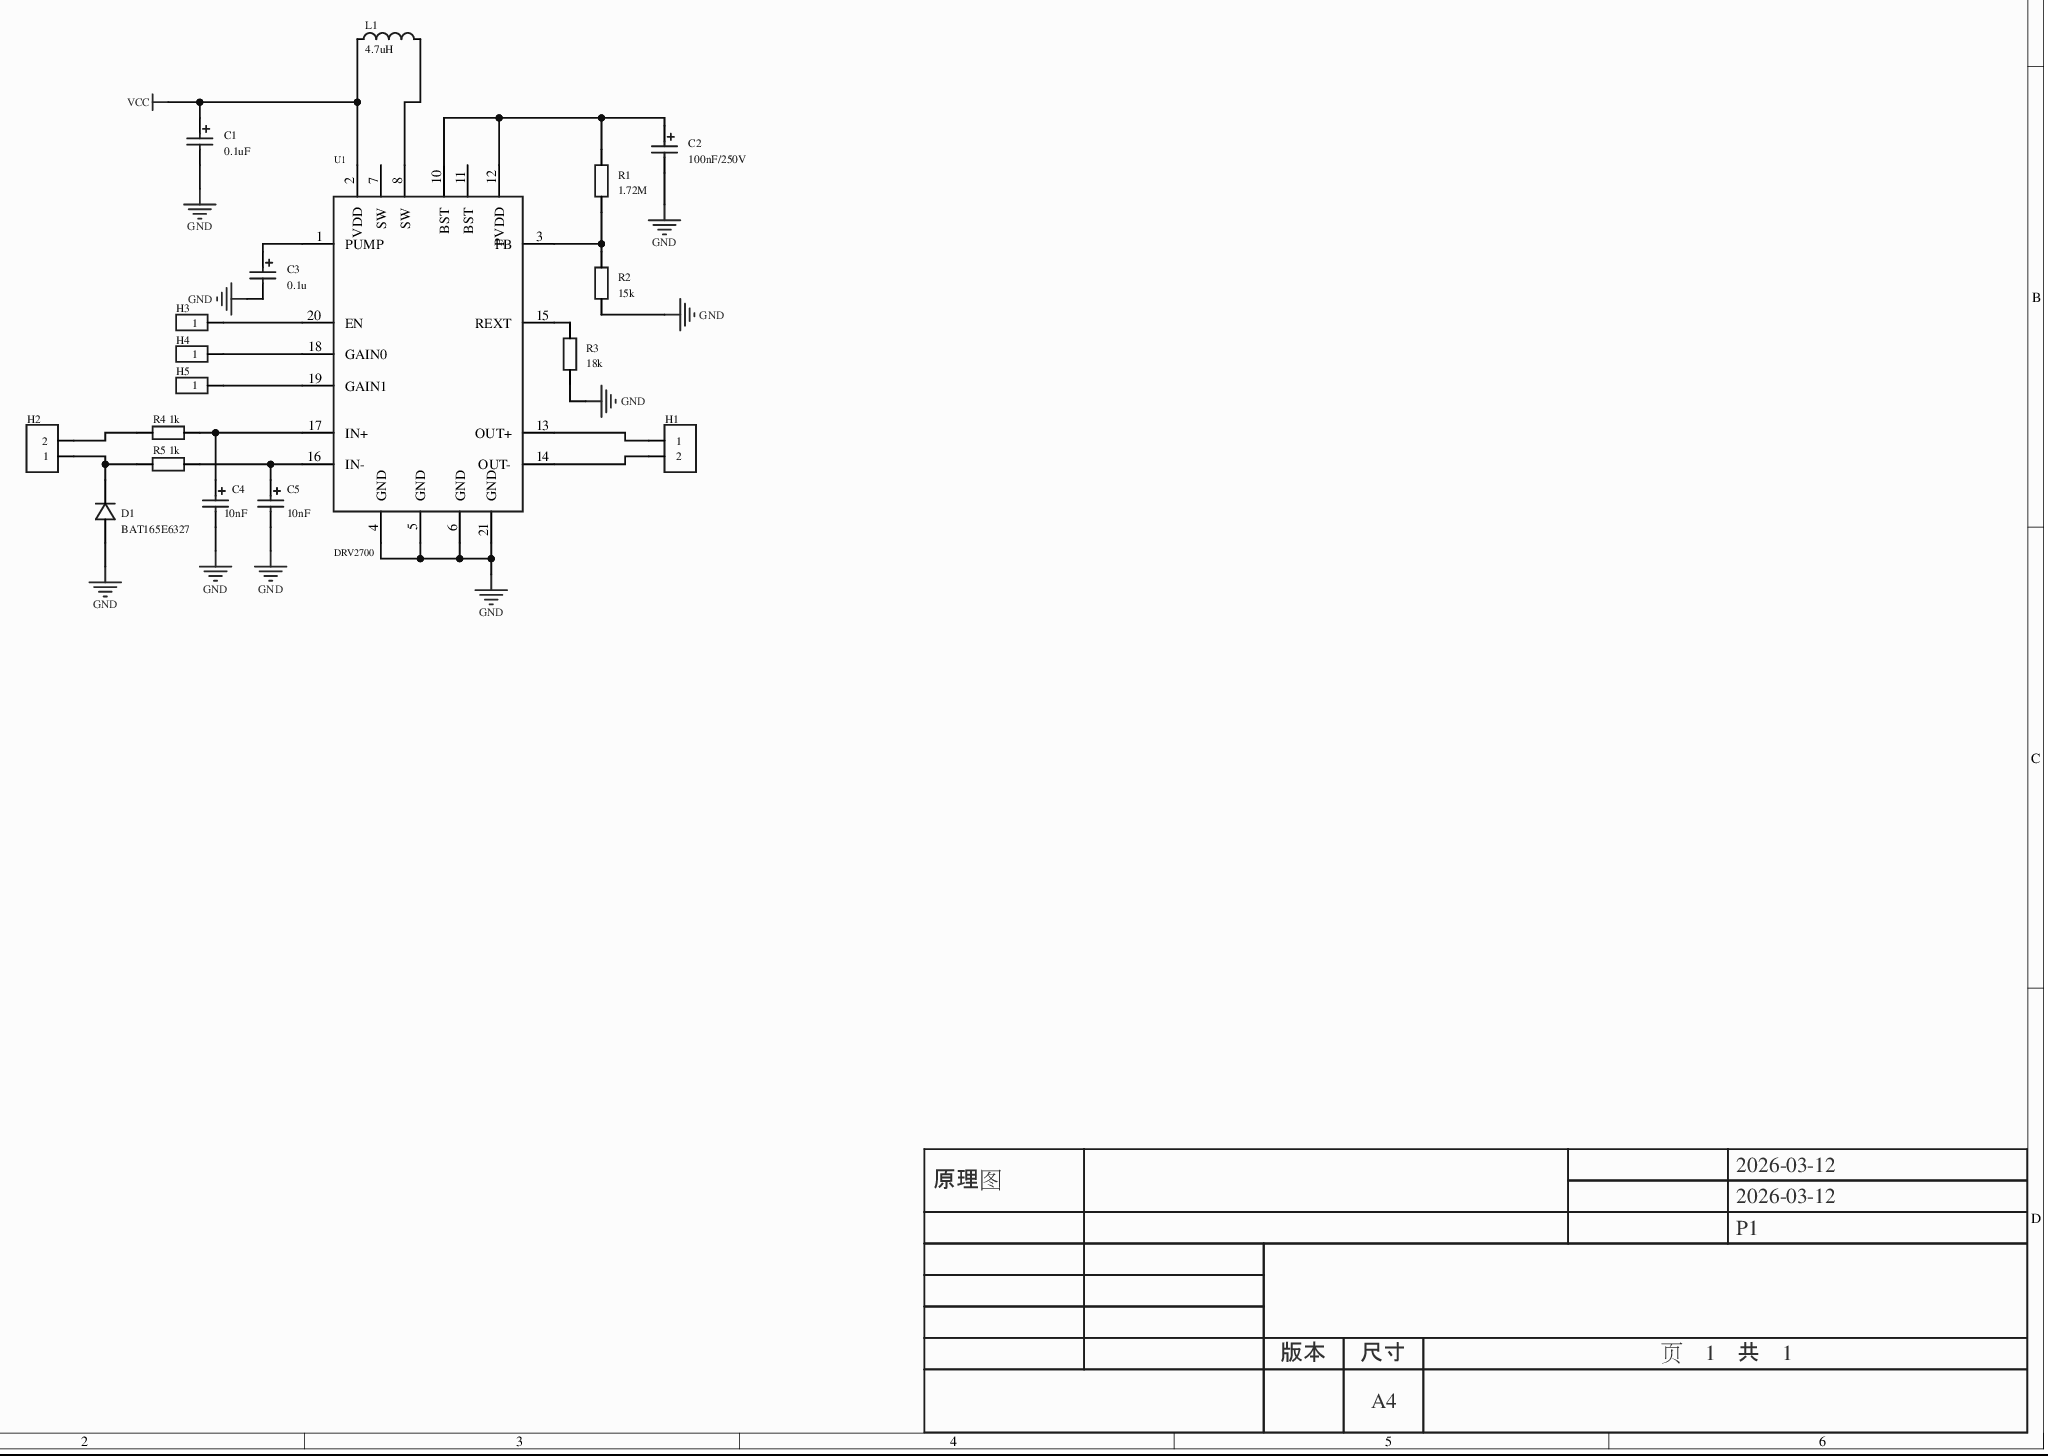
[diagram p0: MISC50934-3.schdoc]
# Altium project MISC50934-2.PrjPcb
1 sheet, 18 parts. Net scope: global (net labels, ports and power ports of the same name join across sheets).
Board file: MISC50934.pcbdoc

## Sheet MISC50934-3.schdoc
size 420 x 297 mm; Version: V1.0; @Project Name: MISC50934; @Update Date: 2026-03-12; @Create Date: 2026-03-12; @Board Name: MISC50934; @Create Time: 20:29:02; @Page Count: 1; @Page No: 1; @Schematic Name: MISC50934; @Update Time: 20:29:02; Size: A4

### Parts
C1  0.1uF  [C_Ele_SMD_3x5.4mm]
C2  100nF/250V  [C_Ele_SMD_3x5.4mm]
C3  0.1u  [C_Ele_SMD_3x5.4mm]
C4  10nF  [C_Ele_SMD_3x5.4mm]
C5  10nF  [C_Ele_SMD_3x5.4mm]
D1  BAT165E6327  [SOD-323_L1.8-W1.3-LS2.5-RD]
H1  (no value)  [HDR-TH_2P-P2.54-V-F]
H2  (no value)  [HDR-TH_2P-P2.54-V-F]
H3  (no value)  [HDR-TH_1P-V-M_XKB_X4611WV-01I-C28D40]
H4  (no value)  [HDR-TH_1P-V-M_XKB_X4611WV-01I-C28D40]
H5  (no value)  [HDR-TH_1P-V-M_XKB_X4611WV-01I-C28D40]
L1  4.7uH  [IND-SMD_L4.6-W4.1-A]
R1  1.72M  [Res_1W]
R2  15k  [Res_1W]
R3  18k  [Res_1W]
R4  1k  [Res_1W]
R5  1k  [Res_1W]
U1  DRV2700  [TI-RGP20-2700X2700TP_V]

### Nets
GND: C1.2 C2.2 C3.2 C4.2 C5.2 D1.2(A) R2.1 R3.1 U1.4(GND) U1.5(GND) U1.6(GND) U1.21(GND)
VCC: C1.1 L1.1 U1.2(VDD)
NetC2_1: C2.1 R1.2 U1.10(BST) U1.12(PVDD)
NetC3_1: C3.1 U1.1(PUMP)
NetC4_1: C4.1 R4.2 U1.17(IN+)
NetC5_1: C5.1 R5.2 U1.16(IN-)
NetD1_1: D1.1(C) H2.1 R5.1
NetH1_1: H1.1 U1.13(OUT+)
NetH1_2: H1.2 U1.14(OUT-)
NetH2_2: H2.2 R4.1
NetH3_1: H3.1 U1.20(EN)
NetH4_1: H4.1 U1.18(GAIN0)
NetH5_1: H5.1 U1.19(GAIN1)
NetL1_2: L1.2 U1.8(SW)
NetR1_1: R1.1 R2.2 U1.3(FB)
NetR3_2: R3.2 U1.15(REXT)

Not connected (* = marked no-connect by the designer): U1 7(SW)* 11(BST)*

### Notes on the sheet
- 2026-03-12
- 原理图
- P1
- 版本
- 尺寸
- A4
- 页    1    共    1

### Library data of the parts
C1-C5 = C_Ele_SMD_3x5.4mm: Symbol: CAP; AddInBom: yes; ModelId: 0132c3d3fdbf4fd987f710a97e7a5b5d0819f05c4eef4c71ace90d822a990e87; ModelName: CAP-SMD_BD3.0-L3.3-W3.3-H5.3; ModelTransform: 129.9,149.58,209.06,-90,0,0,0,0,0; Device: C_Ele_SMD_3x5.4mm; FootprintName: C_Ele_SMD_3x5.4mm; Supplier Footprint: SMD,3x5.4mm; ConvertToPcb: yes
  C1: Value: 0.1uF
  C2: Value: 100nF/250V
  C3: Value: 0.1u
  C4 C5: Value: 10nF
D1 = BAT165E6327: 二极管配置:1个独立式;正向压降(Vf):740mV@750mA;直流反向耐压(Vr):40V;整流电流:750mA;; Manufacturer: Infineon(英飞凌); Symbol: BAT165E6327HTSA1; AddInBom: yes; Diode Configuration: 1个独立式; Voltage - DC Reverse(Vr): 40V; Current - Rectified: 750mA; Reverse Leakage Current (Ir): 50uA@40V; Non-Repetitive Peak Forward Surge Current: 2.5A; ModelId: 7459fe65e23146c0a8d836e46a0add720819f05c4eef4c71ace90d822a990e87; ModelTransform: 104.3305,51.181,0,0,0,0,0,0,0; Device: BAT165E6327; FootprintName: SOD-323_L1.8-W1.3-LS2.5-RD; LCSC Part Name: 电压:40V 电流:750mA; SupplierPart: C151511; ManufacturerPart: BAT165E6327; Supplier Footprint: SOD-323; JLCPCB Part Class: Extended Part; Datasheet: https://item.szlcsc.com/datasheet/BAT165E6327/162851.html; Supplier: LCSC; ConvertToPcb: yes; Voltage - Forward(Vf@If): 740mV@750mA; ModelName: SOD-323_L1.8-W1.3-LS2.5-RD
H1 H2 = HDR-F_2.54_1x2P: Symbol: Header-Female-2.54_1x2; ConvertToPcb: yes; ModelId: a9450ef445564560a104363b9aacde4e0819f05c4eef4c71ace90d822a990e87; ModelName: HDR-TH_2P-P2.54-F-LI-1X2P; ModelTransform: 215.7476,98.425,0,0,0,0,0,0,-129.921; Device: HDR-F_2.54_1x2P; FootprintName: HDR-TH_2P-P2.54-V-F; AddInBom: yes; SupplierPart: C49661; Supplier Footprint: 插件
H3-H5 = HDR-M_2.54_1x1P: Symbol: HDR_1x1; ConvertToPcb: yes; ModelId: 95857080d3cc4057a19a22ccce05e1710819f05c4eef4c71ace90d822a990e87; ModelTransform: 78.74,79.1337,0,0,0,0,0,0,-110.236; Device: HDR-M_2.54_1x1P; FootprintName: HDR-TH_1P-V-M_XKB_X4611WV-01I-C28D40; AddInBom: yes; SupplierPart: C81276; Supplier Footprint: 插件; JLCPCB Part Class: Extended Part; ModelName: HDR-TH_1P-V-M_XKB_X4611WV-01I-C28D40
L1 = SRG0420-4R7-M: 电感值:4.7uH;精度:±20%;额定电流:3A;饱和电流(Isat):3.5A;类型:一体成型电感;; Manufacturer: JIERR(捷而瑞); AddInBom: yes; Tolerance: ±20%; Current Rating: 3A; Current - Saturation(Isat): 3.5A; DC Resistance(DCR): 105mΩ; Type: 一体成型电感; ModelId: 3b00517e351145dc8b8e2e52a7e5ed2c0819f05c4eef4c71ace90d822a990e87; ModelName: IND-SMD_L4.6-W4.1-H1.5; ModelTransform: 181.102,161.417,0,0,0,0,0,0,0; Device: SRG0420-4R7-M; Symbol: SRG0420-4R7-M; FootprintName: IND-SMD_L4.6-W4.1-A; LCSC Part Name: 4.7μH ±20% 3.5A; SupplierPart: C53462918; ManufacturerPart: SRG0420-4R7-M; Supplier Footprint: SMD,4.6x4.1mm; JLCPCB Part Class: Extended Part; Datasheet: https://item.szlcsc.com/datasheet/SRG0420-4R7-M/56628163.html; Supplier: LCSC; ConvertToPcb: yes; Value: 4.7uH
R1-R5 = Res_AXIAL-1W: Symbol: 电阻; ConvertToPcb: yes; ModelId: f1f7cfb3d56f4763951150e77c261d090819f05c4eef4c71ace90d822a990e87; ModelName: RES-TH_BD4.5-L11.5-P15.50-D0.8; ModelTransform: 641.71,177.16,374,0,0,0,0,0,-190; Device: Res_AXIAL-1W; FootprintName: Res_1W; AddInBom: yes; Supplier Footprint: 轴向引线
  R1: Value: 1.72M
  R2: Value: 15k
  R3: Value: 18k
  R4 R5: Value: 1k
U1 = DRV2700: Device: DRV2700; Symbol: DRV2700; FootprintName: TI-RGP20-2700X2700TP_V